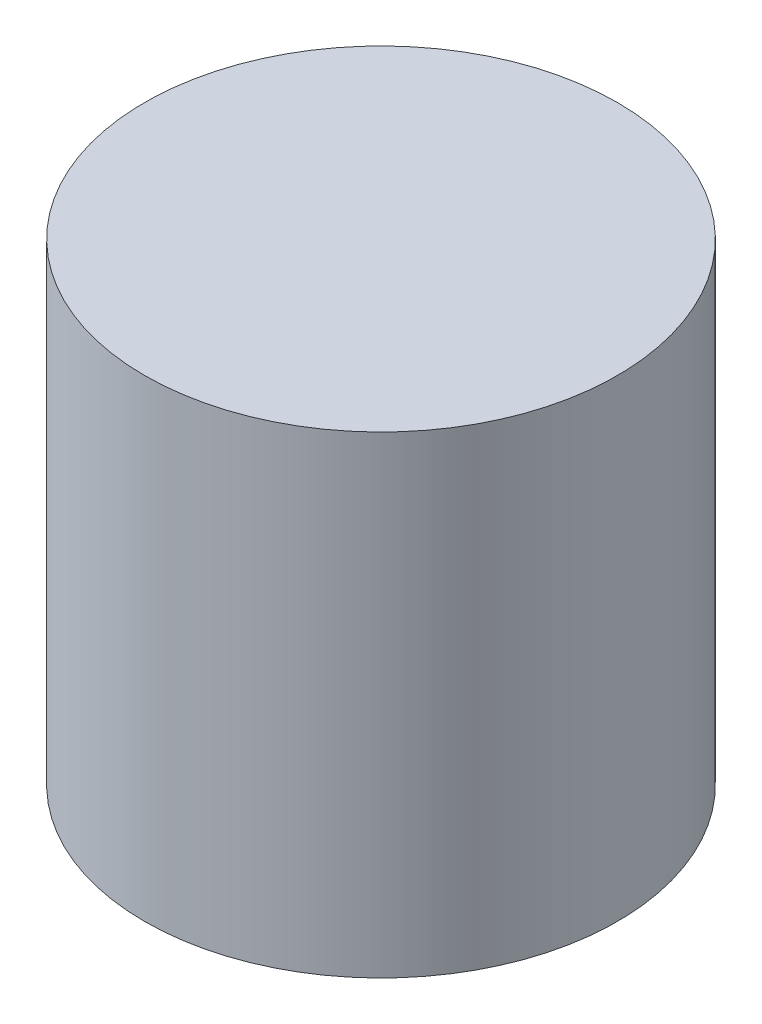
from build123d import *


with BuildPart() as part:
    # Sketch1 → Revolve1 (revolve)
    with BuildSketch(Plane.XY, mode=Mode.PRIVATE) as revolve1_sk:
        Polygon((0, 24.447340426), (10, 24.447340426), (10, 4.447340426), (2.5, 4.447340426), (2.5, 0.447340426), (0, 0.447340426), align=None)
    revolve(revolve1_sk.sketch.rotate(Axis((0, 8.62287234, 0), (0, -1, 0)), 90), axis=Axis((0, 8.62287234, 0), (0, -1, 0)))


solid = part.part
